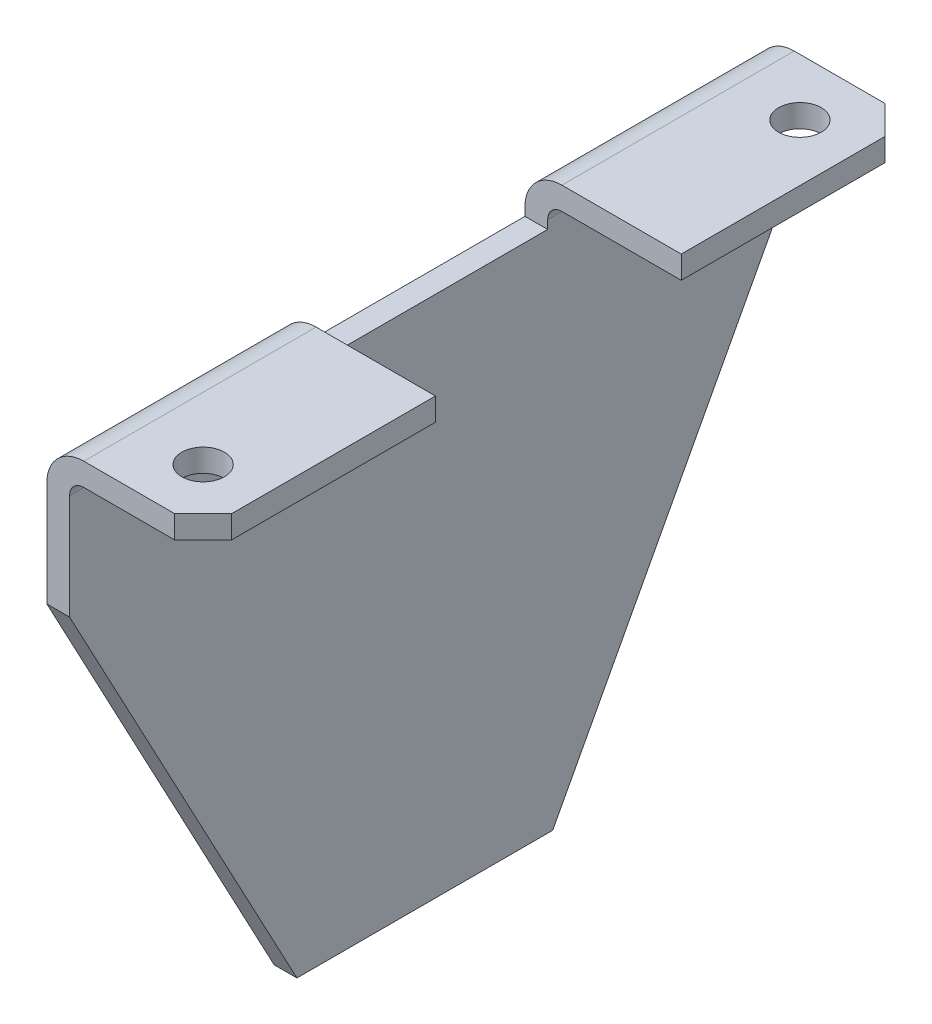
from build123d import *

# Parameters (mm, degrees)
BOSS_EXTRUDE1_DEPTH = 250
SKETCH2_W           = 86.5
SKETCH2_H           = 88.492592909
CUT_EXTRUDE1_DEPTH  = 250
SKETCH3_R           = 7.5
CUT_EXTRUDE2_DEPTH  = 250
CHAMFER1_SIZE       = 10


with BuildPart() as part:
    # Sketch1 → Boss-Extrude1 (new body)
    with BuildSketch(Plane.XY):
        with BuildLine():
            Line((0, 0), (-42, 0))
            ThreePointArc((-42, 0), (-51.192388155, -3.807611845), (-55, -13))
            Line((-55, -13), (-55, -200))
            Line((-55, -200), (-47, -200))
            Line((-47, -200), (-47, -13))
            ThreePointArc((-47, -13), (-45.535533906, -9.464466094), (-42, -8))
            Line((-42, -8), (0, -8))
            Line((0, -8), (0, 0))
        make_face()
    extrude(amount=BOSS_EXTRUDE1_DEPTH)

    # Sketch2 → Cut-Extrude1 (cut)
    with BuildSketch(Plane.ZY.offset(55)):
        Polygon((0, -50), (80, -200), (0, -200), align=None)
        Polygon((170, -200), (250, -200), (250, -50), align=None)
        with Locations((125, 28.246296455)):
            Rectangle(SKETCH2_W, SKETCH2_H)
    extrude(amount=-CUT_EXTRUDE1_DEPTH, mode=Mode.SUBTRACT)

    # Sketch3 → Cut-Extrude2 (cut)
    with BuildSketch(Plane(origin=(0, 0, 0), x_dir=(1, 0, 0), z_dir=(0, 1, 0))):
        with Locations(Location((-20, -20, 0), (0, 0, 180))):
            Circle(SKETCH3_R)
        with Locations(Location((-20, -230, 0), (0, 0, 180))):
            Circle(SKETCH3_R)
    extrude(amount=-CUT_EXTRUDE2_DEPTH, mode=Mode.SUBTRACT)

    # Chamfer1
    chamfer1_edges = [part.edges().sort_by_distance(p)[0] for p in [
        (0, -4, 250),
        (0, -4, 0),
    ]]
    chamfer(chamfer1_edges, length=CHAMFER1_SIZE)


solid = part.part
